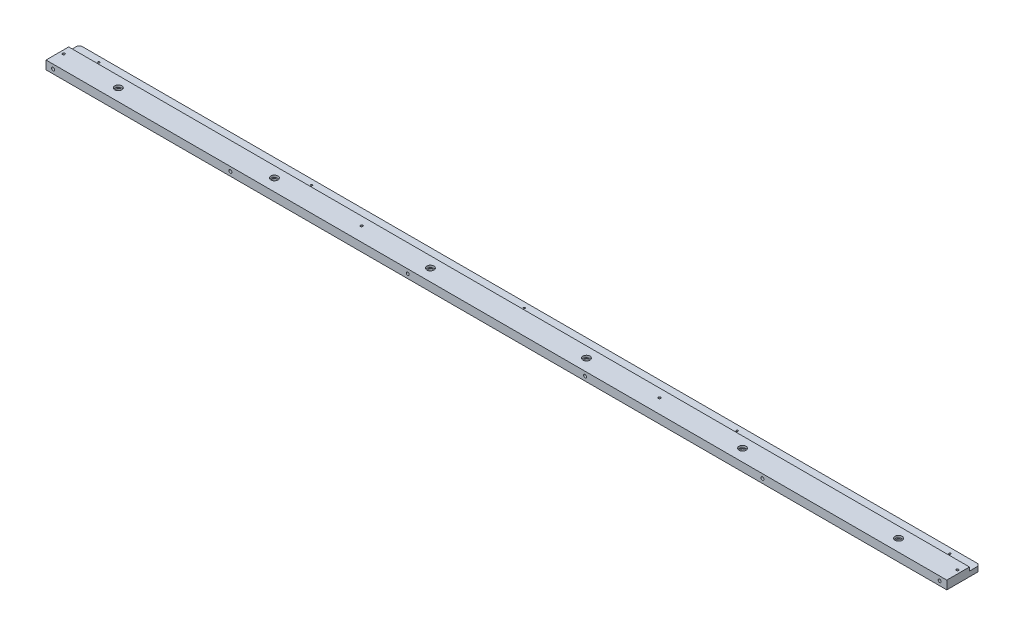
from build123d import *

# Parameters (mm, degrees)
SKETCH_1_W             = 1270
SKETCH_1_H             = 47
EXTRUDE_1_DEPTH        = 6
SKETCH_2_W             = 15
SKETCH_2_H             = 5
CUT_EXTRUDE_1_DEPTH    = 1271.231573376
CHAMFER_1_SIZE         = 3
HOLE_WIZARD_M5_1_D     = 4.2
HOLE_WIZARD_M5_1_DEPTH = 12.4
HOLE_WIZARD_M5_1_TIP   = 1.2618073
HOLE_WIZARD_M4_1_D     = 3.3
HOLE_WIZARD_M3_1_D     = 2.5
HOLE_WIZARD_M8_1_D     = 6.8
SKETCH_12_R            = 5
CUT_EXTRUDE_2_DEPTH    = 3


with BuildPart() as part:
    # 草图1 → 凸台-拉伸1 (new, symmetric)
    with BuildSketch(Plane(origin=(0, 0, 0), x_dir=(1, 0, 0), z_dir=(0, 1, 0))):
        Rectangle(SKETCH_1_W, SKETCH_1_H)
    extrude(amount=EXTRUDE_1_DEPTH, both=True)

    # 草图2 → 切除-拉伸1 (cut, through all)
    with BuildSketch(Plane(origin=(635, 0, 0), x_dir=(0, 0, -1), z_dir=(1, 0, 0))):
        with Locations((16, 3.5)):
            Rectangle(SKETCH_2_W, SKETCH_2_H)
    extrude(amount=-CUT_EXTRUDE_1_DEPTH, mode=Mode.SUBTRACT)

    # 倒角1
    chamfer_1_edges = [part.edges().sort_by_distance(p)[0] for p in [
        (-635, -2.5, -23.5),
        (635, -2.5, -23.5),
    ]]
    chamfer(chamfer_1_edges, length=CHAMFER_1_SIZE)

    # M5 螺纹孔1
    with Locations(Plane.XY.offset(23.5)):
        with Locations((-625, 0), (-375, 0), (-125, 0), (125, 0), (375, 0), (625, 0)):
            Hole(HOLE_WIZARD_M5_1_D / 2, depth=HOLE_WIZARD_M5_1_DEPTH)
            with Locations((0, 0, -(HOLE_WIZARD_M5_1_DEPTH + HOLE_WIZARD_M5_1_TIP / 2))):  # 118° drill point
                Cone(0, HOLE_WIZARD_M5_1_D / 2, HOLE_WIZARD_M5_1_TIP, mode=Mode.SUBTRACT)

    # M4 螺纹孔1 (through all)
    with Locations(Plane(origin=(0, 6, 0), x_dir=(1, 0, 0), z_dir=(0, 1, 0))):
        with Locations((630, -3.5), (-630, -3.5), (210, -3.5), (-210, -3.5)):
            Hole(HOLE_WIZARD_M4_1_D / 2)

    # M3 螺纹孔1 (through all)
    with Locations(Plane(origin=(0, -6, 0), x_dir=(-1, 0, 0), z_dir=(0, -1, 0))):
        with Locations((-600, 16), (-300, 16), (0, 16), (300, 16), (600, 16)):
            Hole(HOLE_WIZARD_M3_1_D / 2)

    # M8 螺纹孔1 (through all)
    with Locations(Plane.XZ.offset(6)):
        with Locations((550, 6.5), (330, 6.5), (110, 6.5), (-110, 6.5), (-330, 6.5), (-550, 6.5)):
            Hole(HOLE_WIZARD_M8_1_D / 2)

    # 草图12 → 切除-拉伸2 (cut)
    with BuildSketch(Plane(origin=(0, 6, 0), x_dir=(1, 0, 0), z_dir=(0, 1, 0))):
        with Locations(Location((550, -6.5, 0), (0, 0, 270))):
            Circle(SKETCH_12_R)
        with Locations(Location((330, -6.5, 0), (0, 0, 270))):
            Circle(SKETCH_12_R)
        with Locations(Location((110, -6.5, 0), (0, 0, 270))):
            Circle(SKETCH_12_R)
        with Locations(Location((-110, -6.5, 0), (0, 0, 270))):
            Circle(SKETCH_12_R)
        with Locations(Location((-330, -6.5, 0), (0, 0, 270))):
            Circle(SKETCH_12_R)
        with Locations(Location((-550, -6.5, 0), (0, 0, 270))):
            Circle(SKETCH_12_R)
    extrude(amount=-CUT_EXTRUDE_2_DEPTH, mode=Mode.SUBTRACT)


solid = part.part
